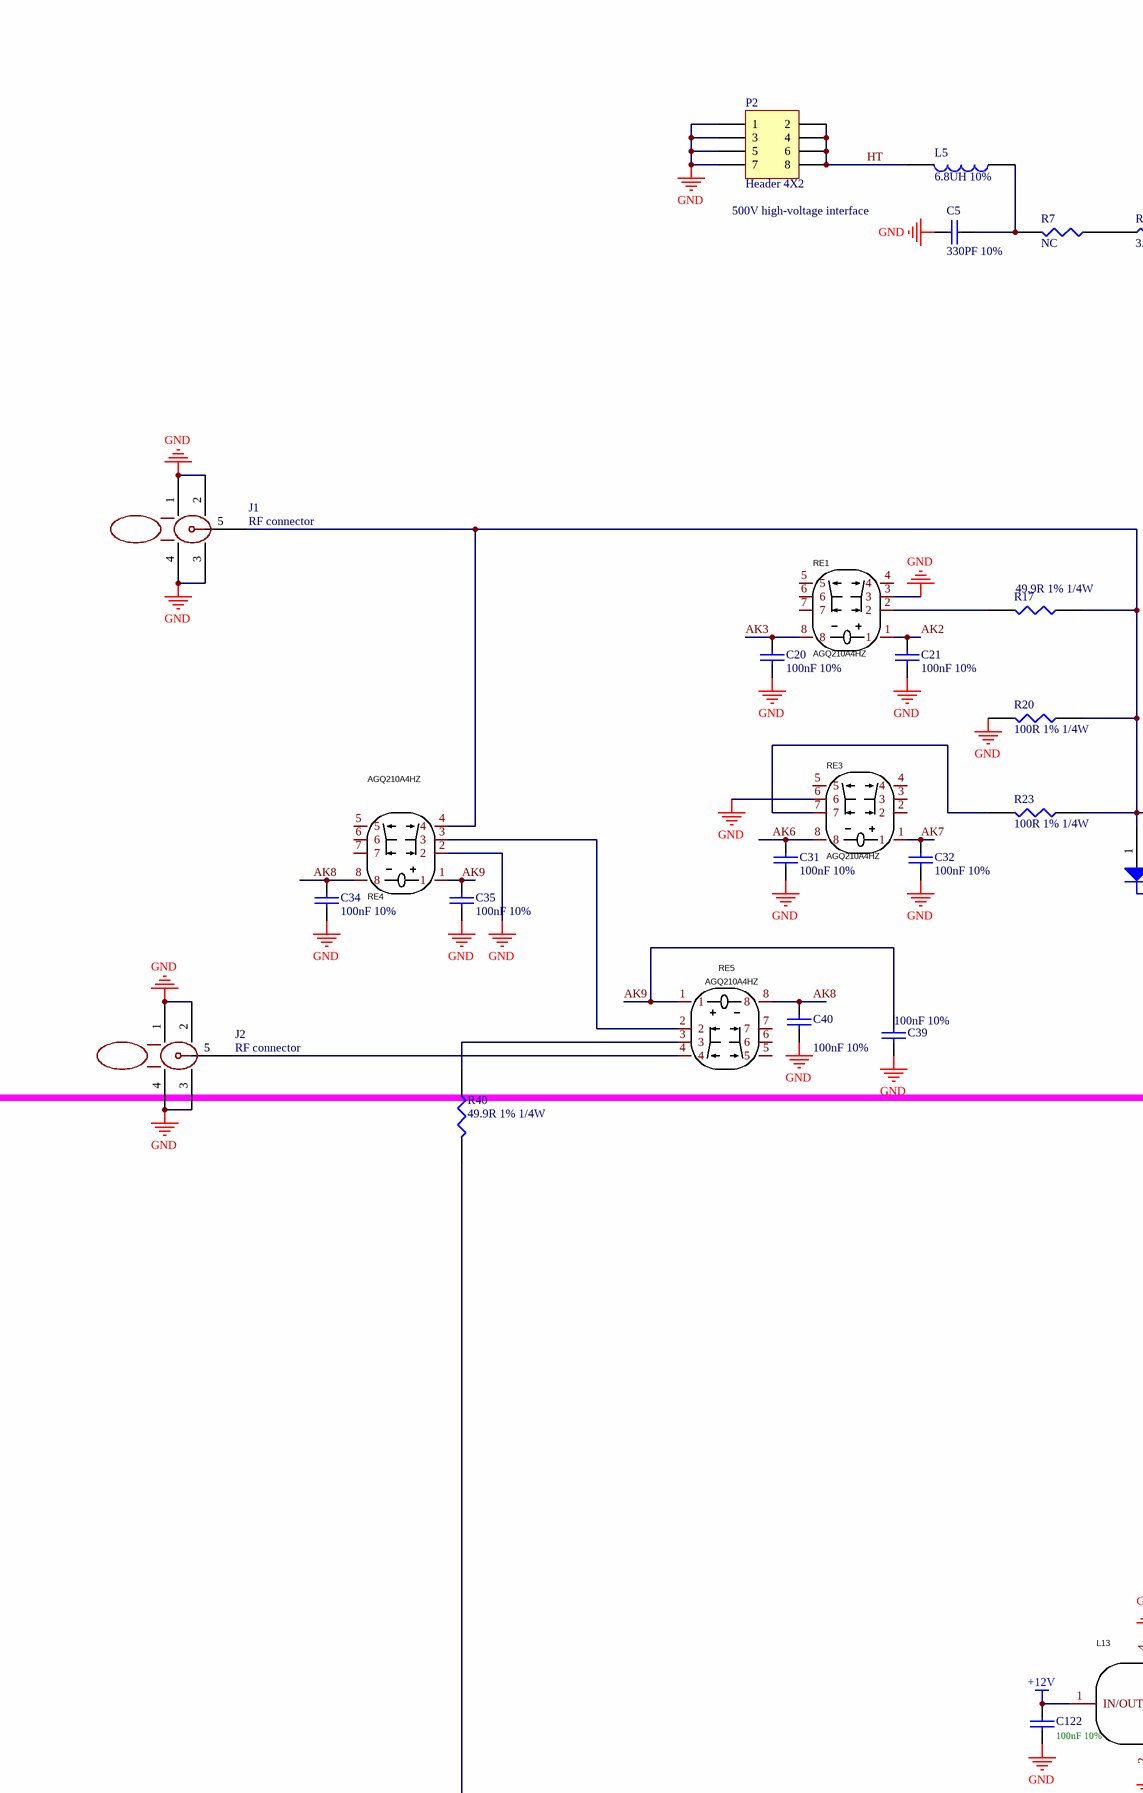
[diagram p0: PCBE109560-12.SchDoc, top left]
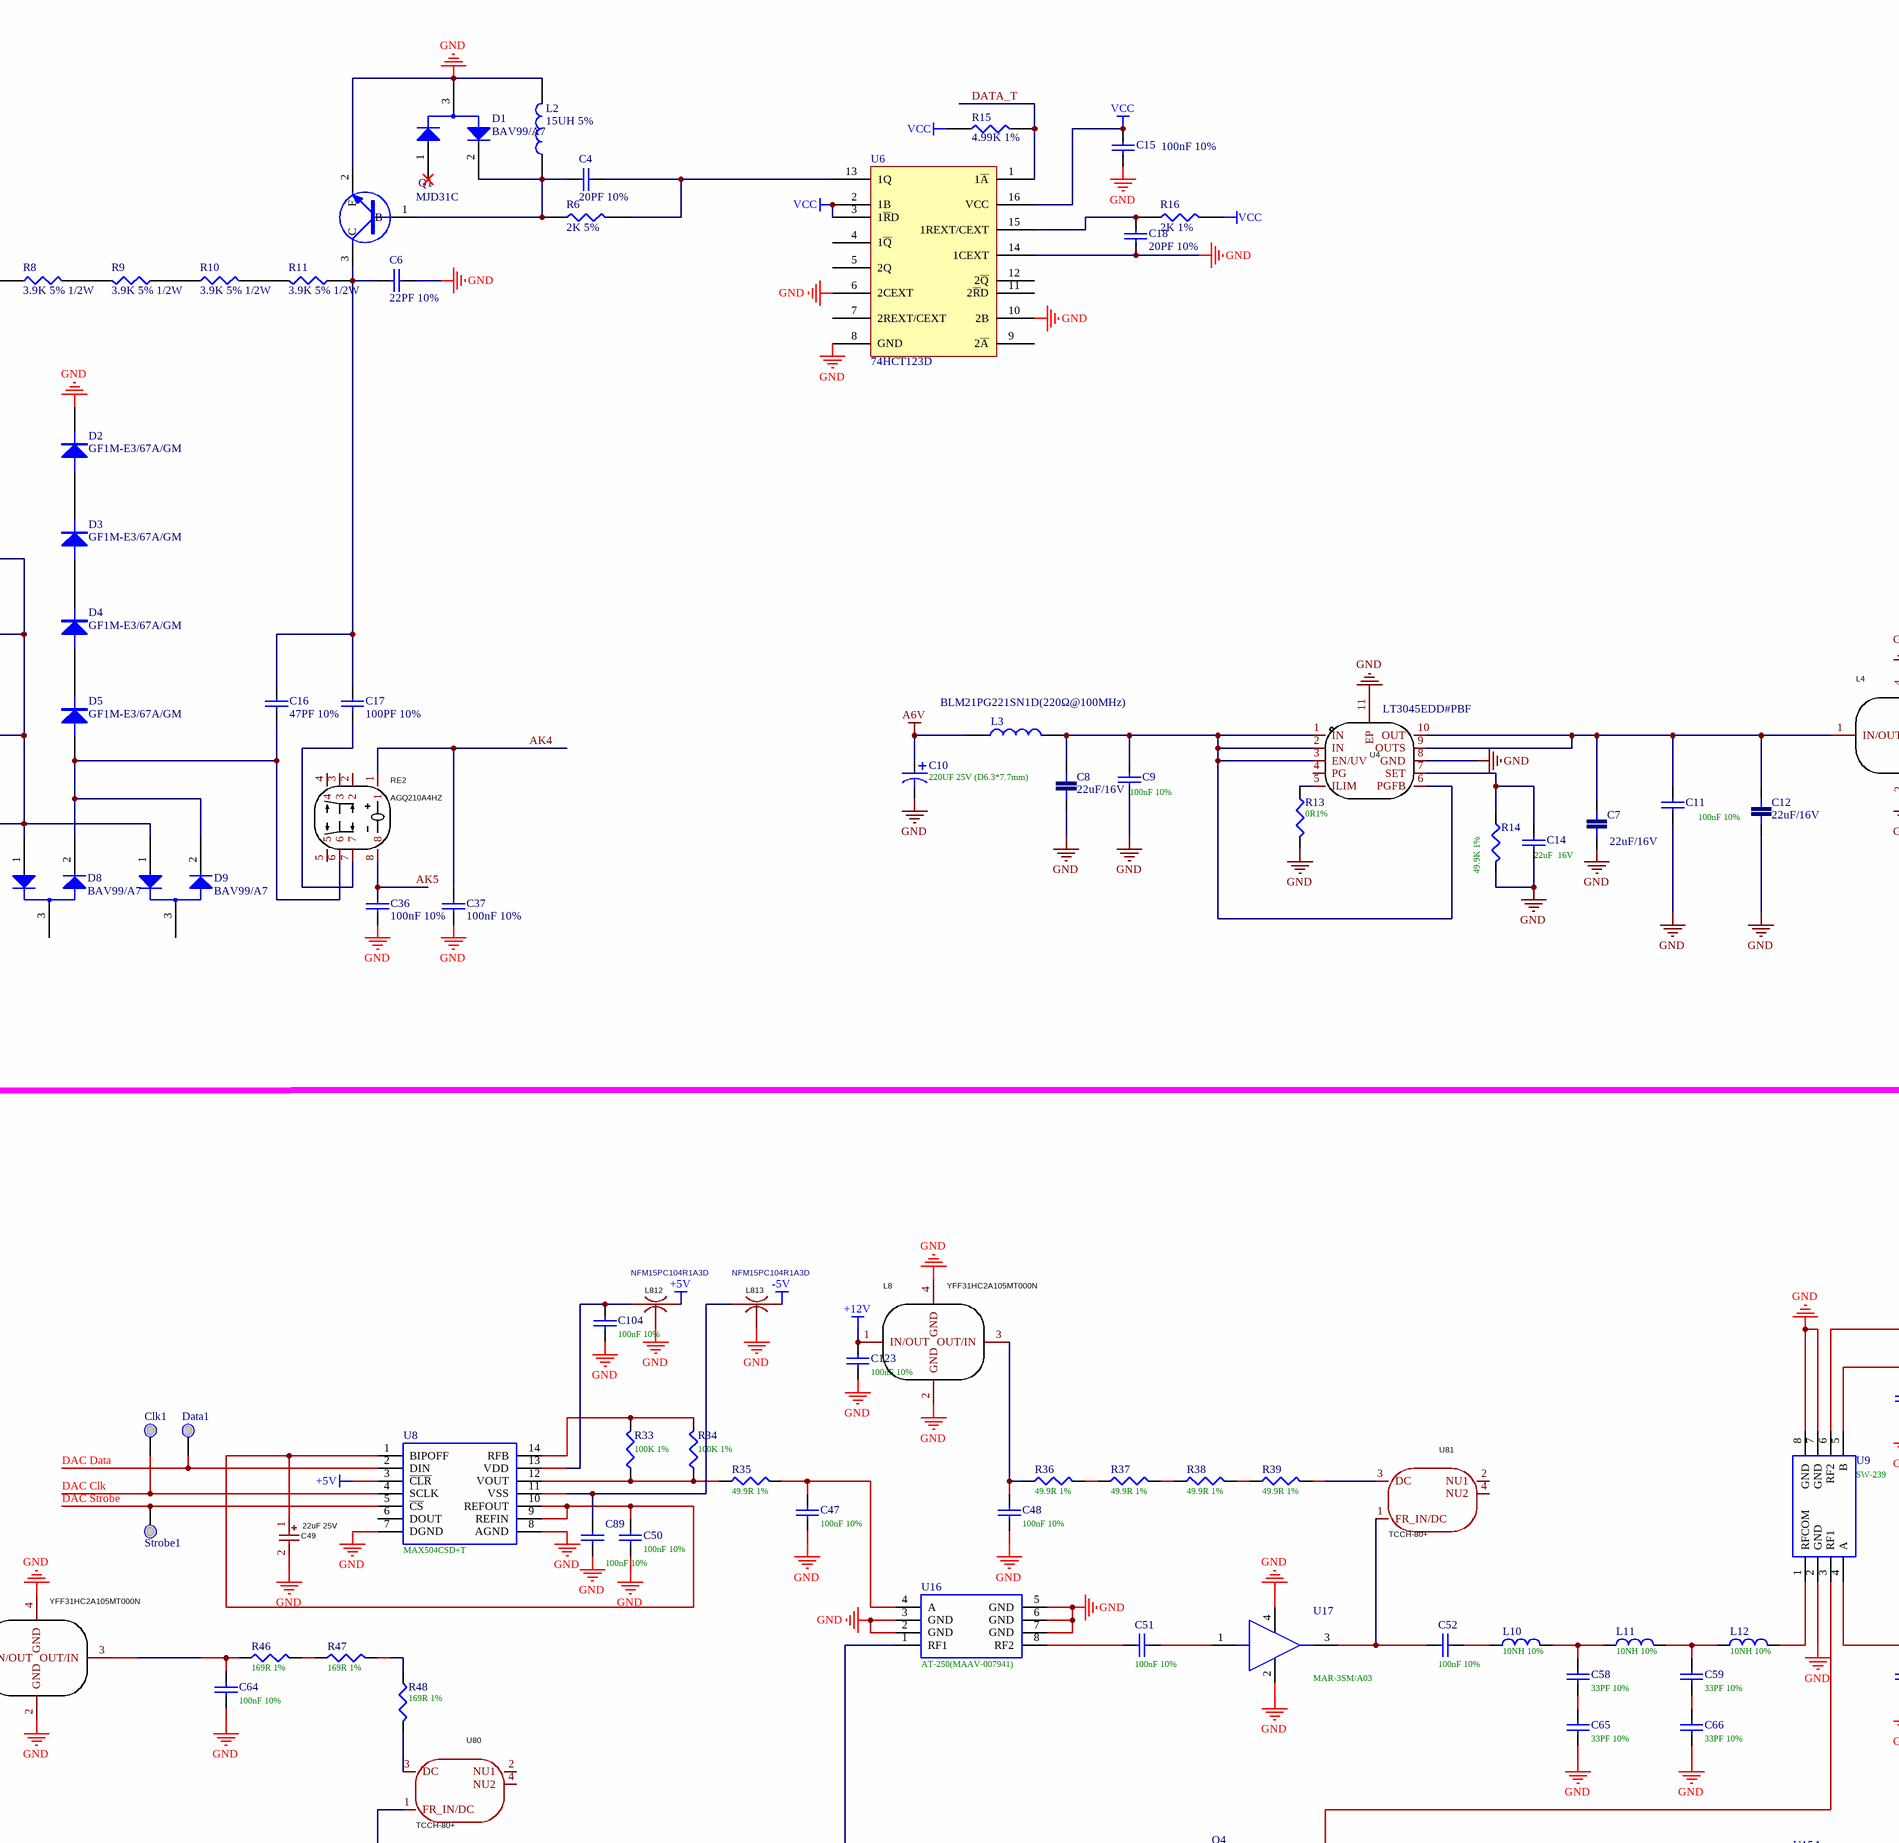
[diagram p1: PCBE109560-12.SchDoc, top middle]
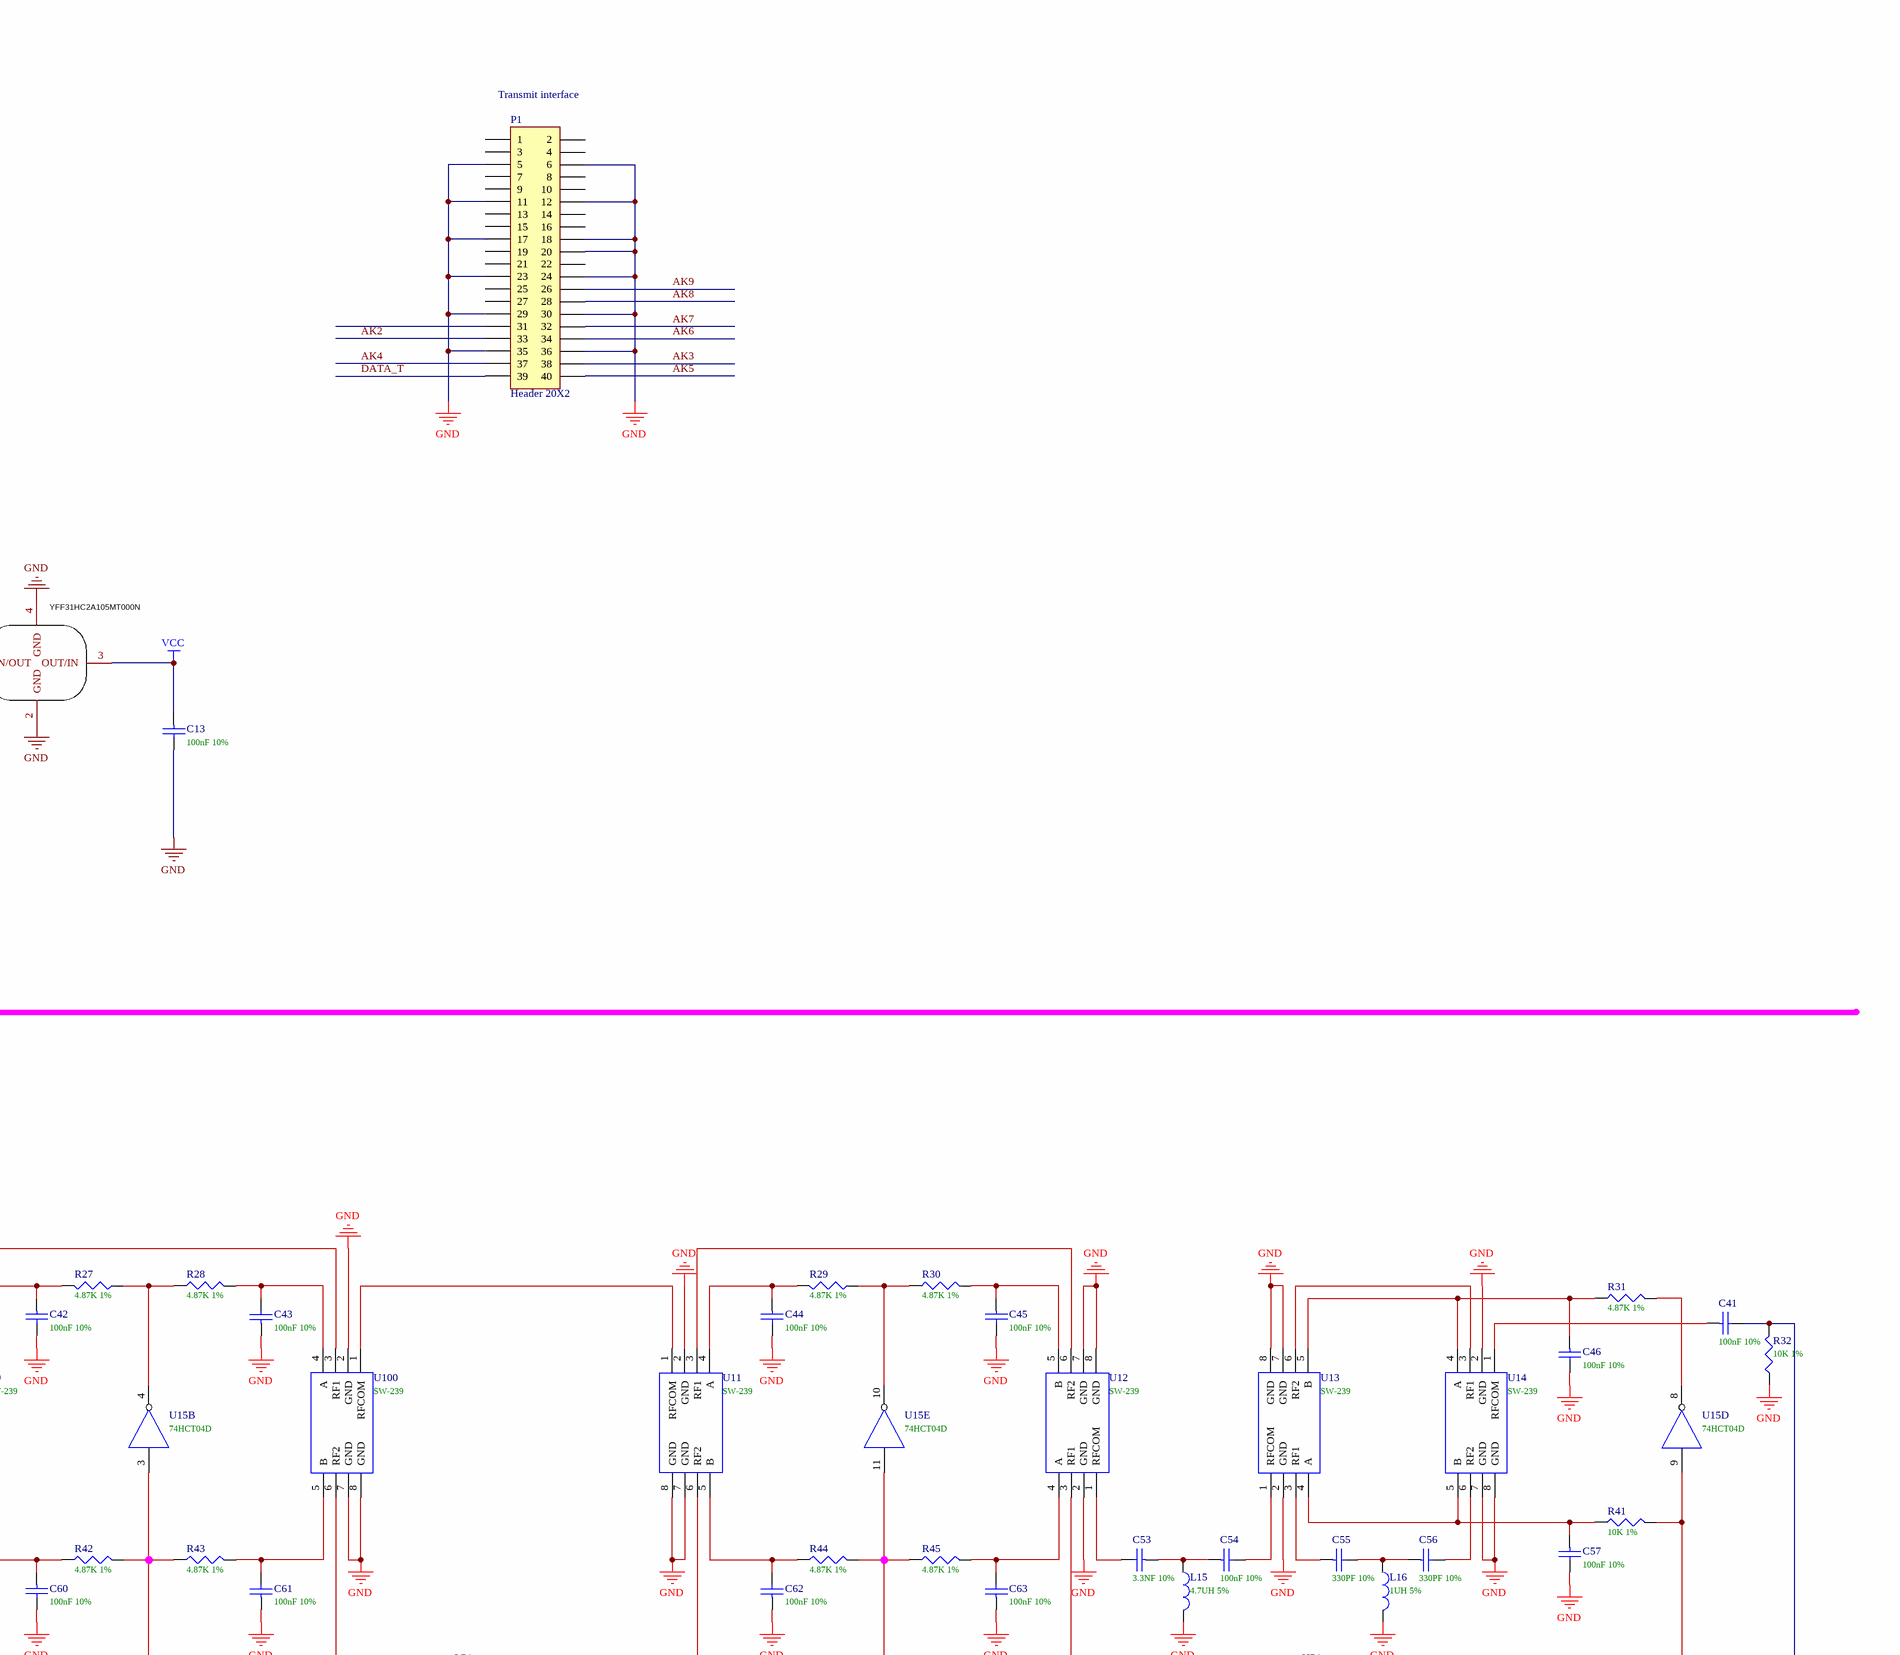
[diagram p2: PCBE109560-12.SchDoc, top right]
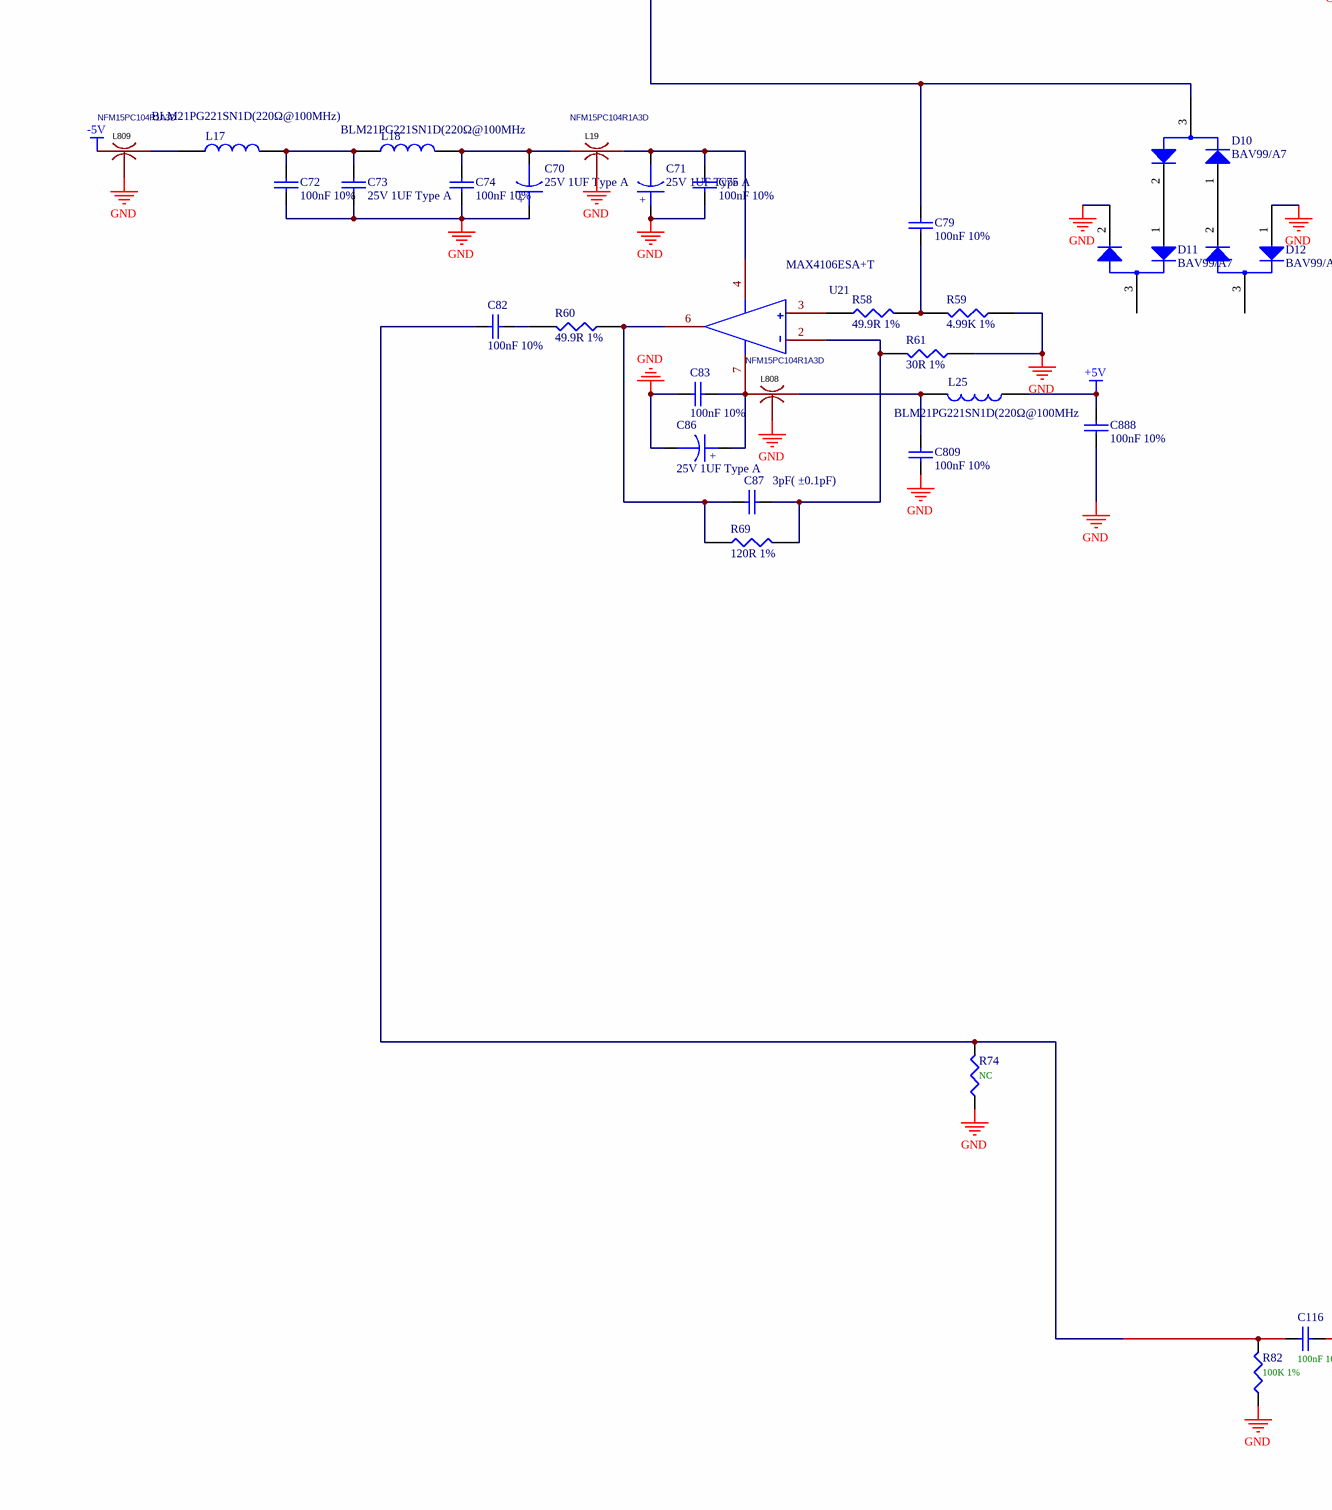
[diagram p3: PCBE109560-12.SchDoc, bottom left]
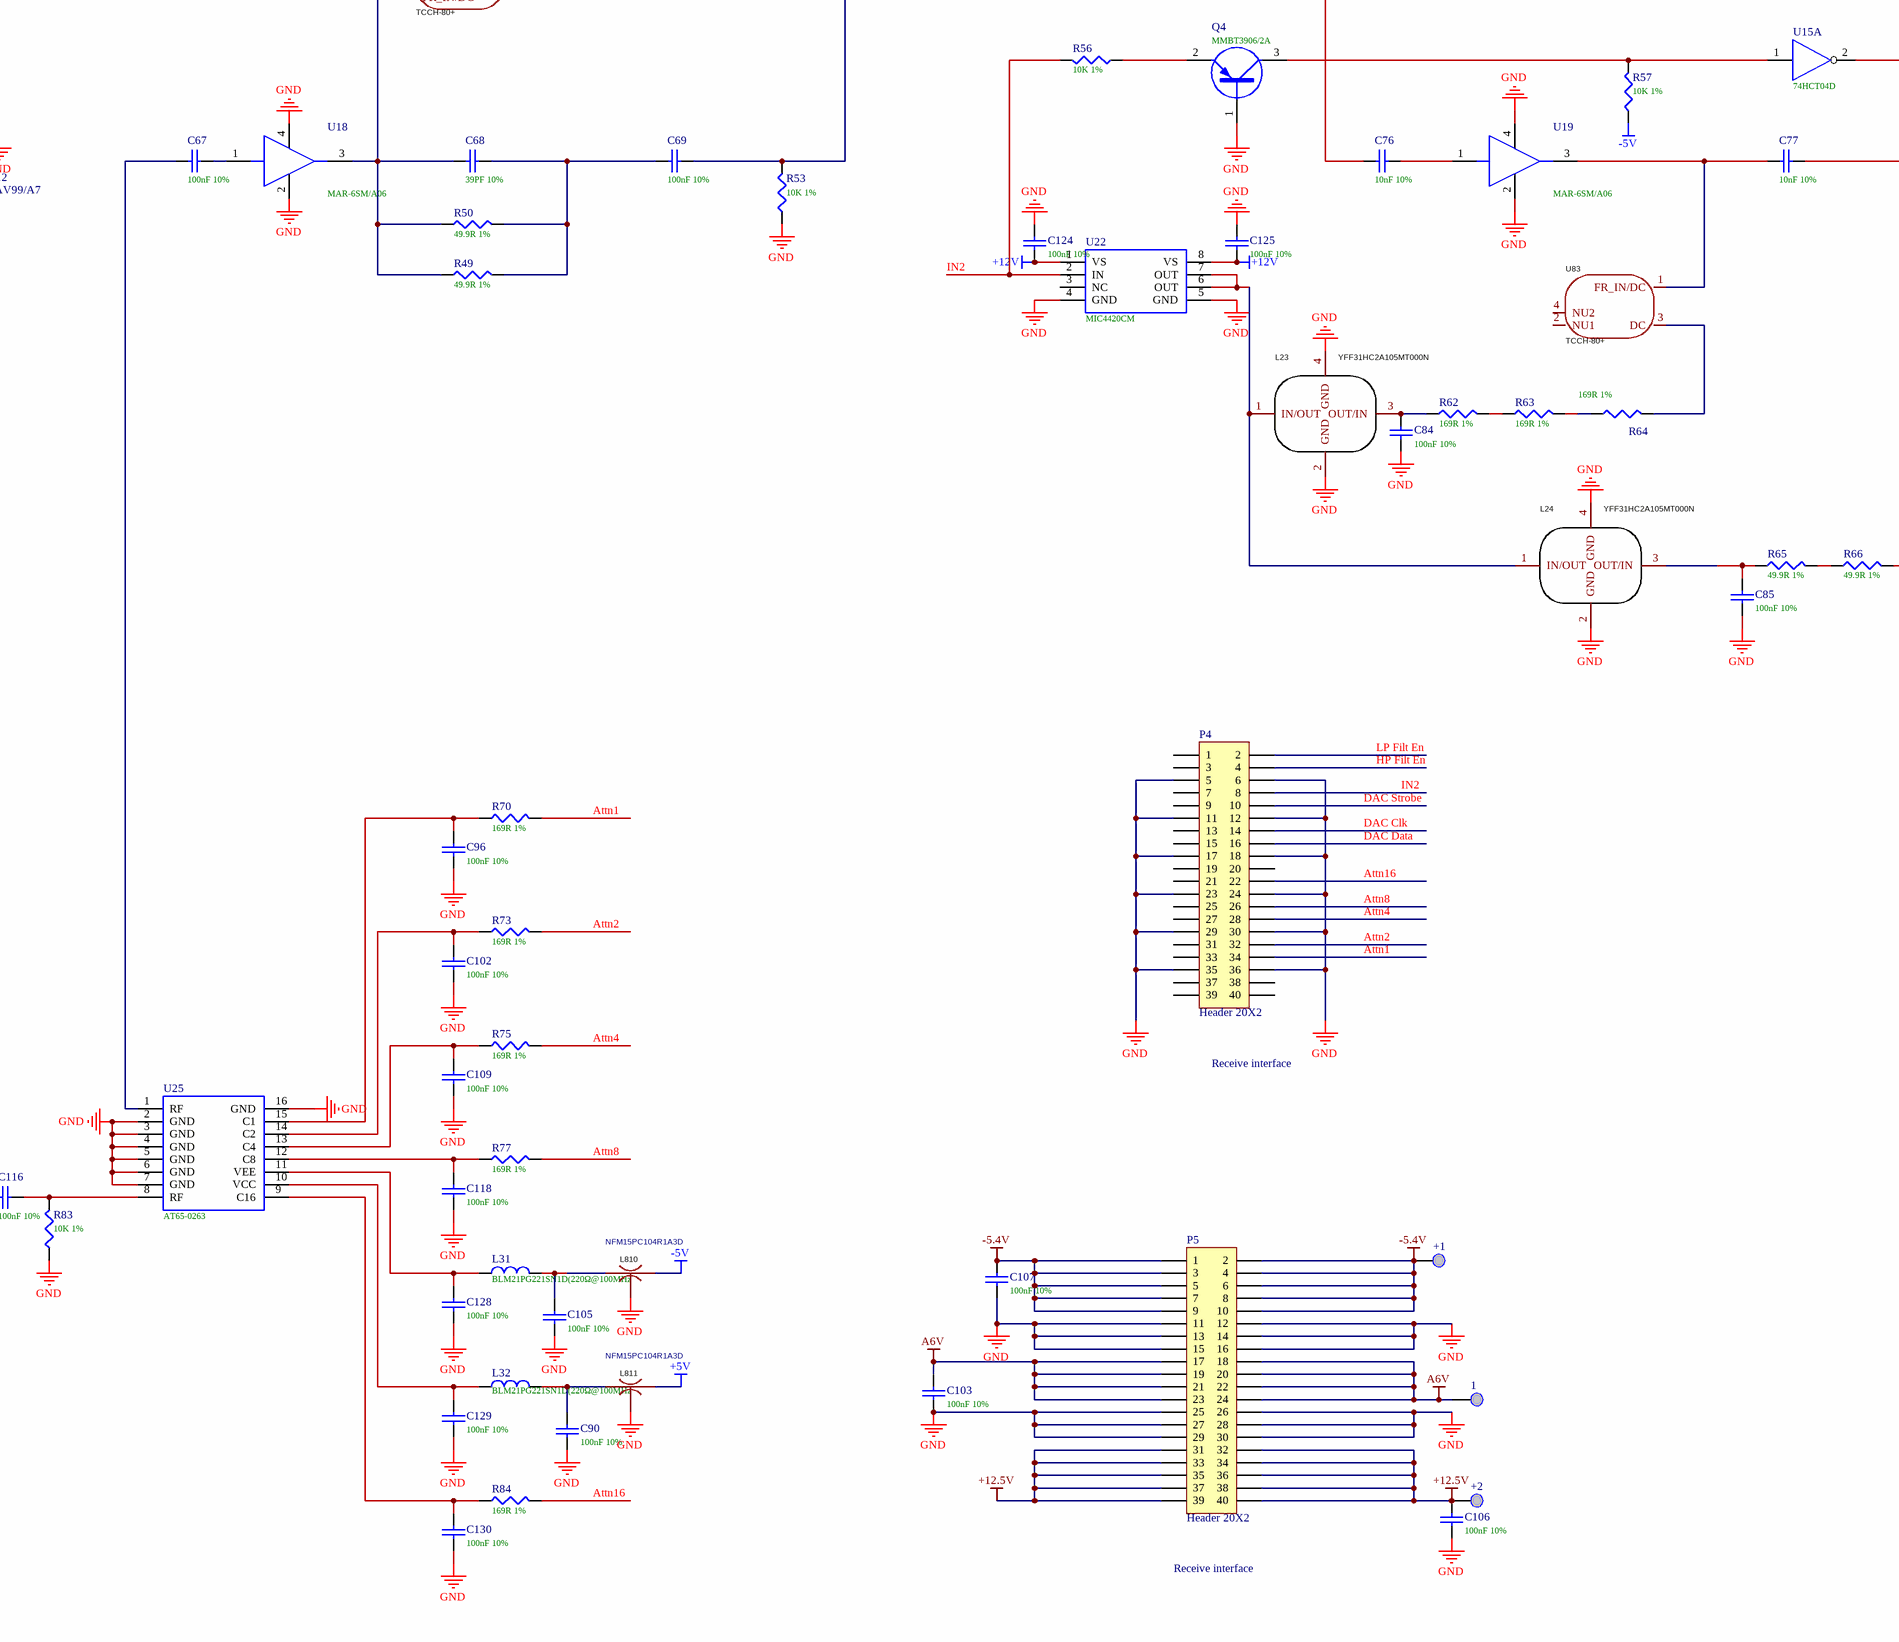
[diagram p4: PCBE109560-12.SchDoc, bottom middle]
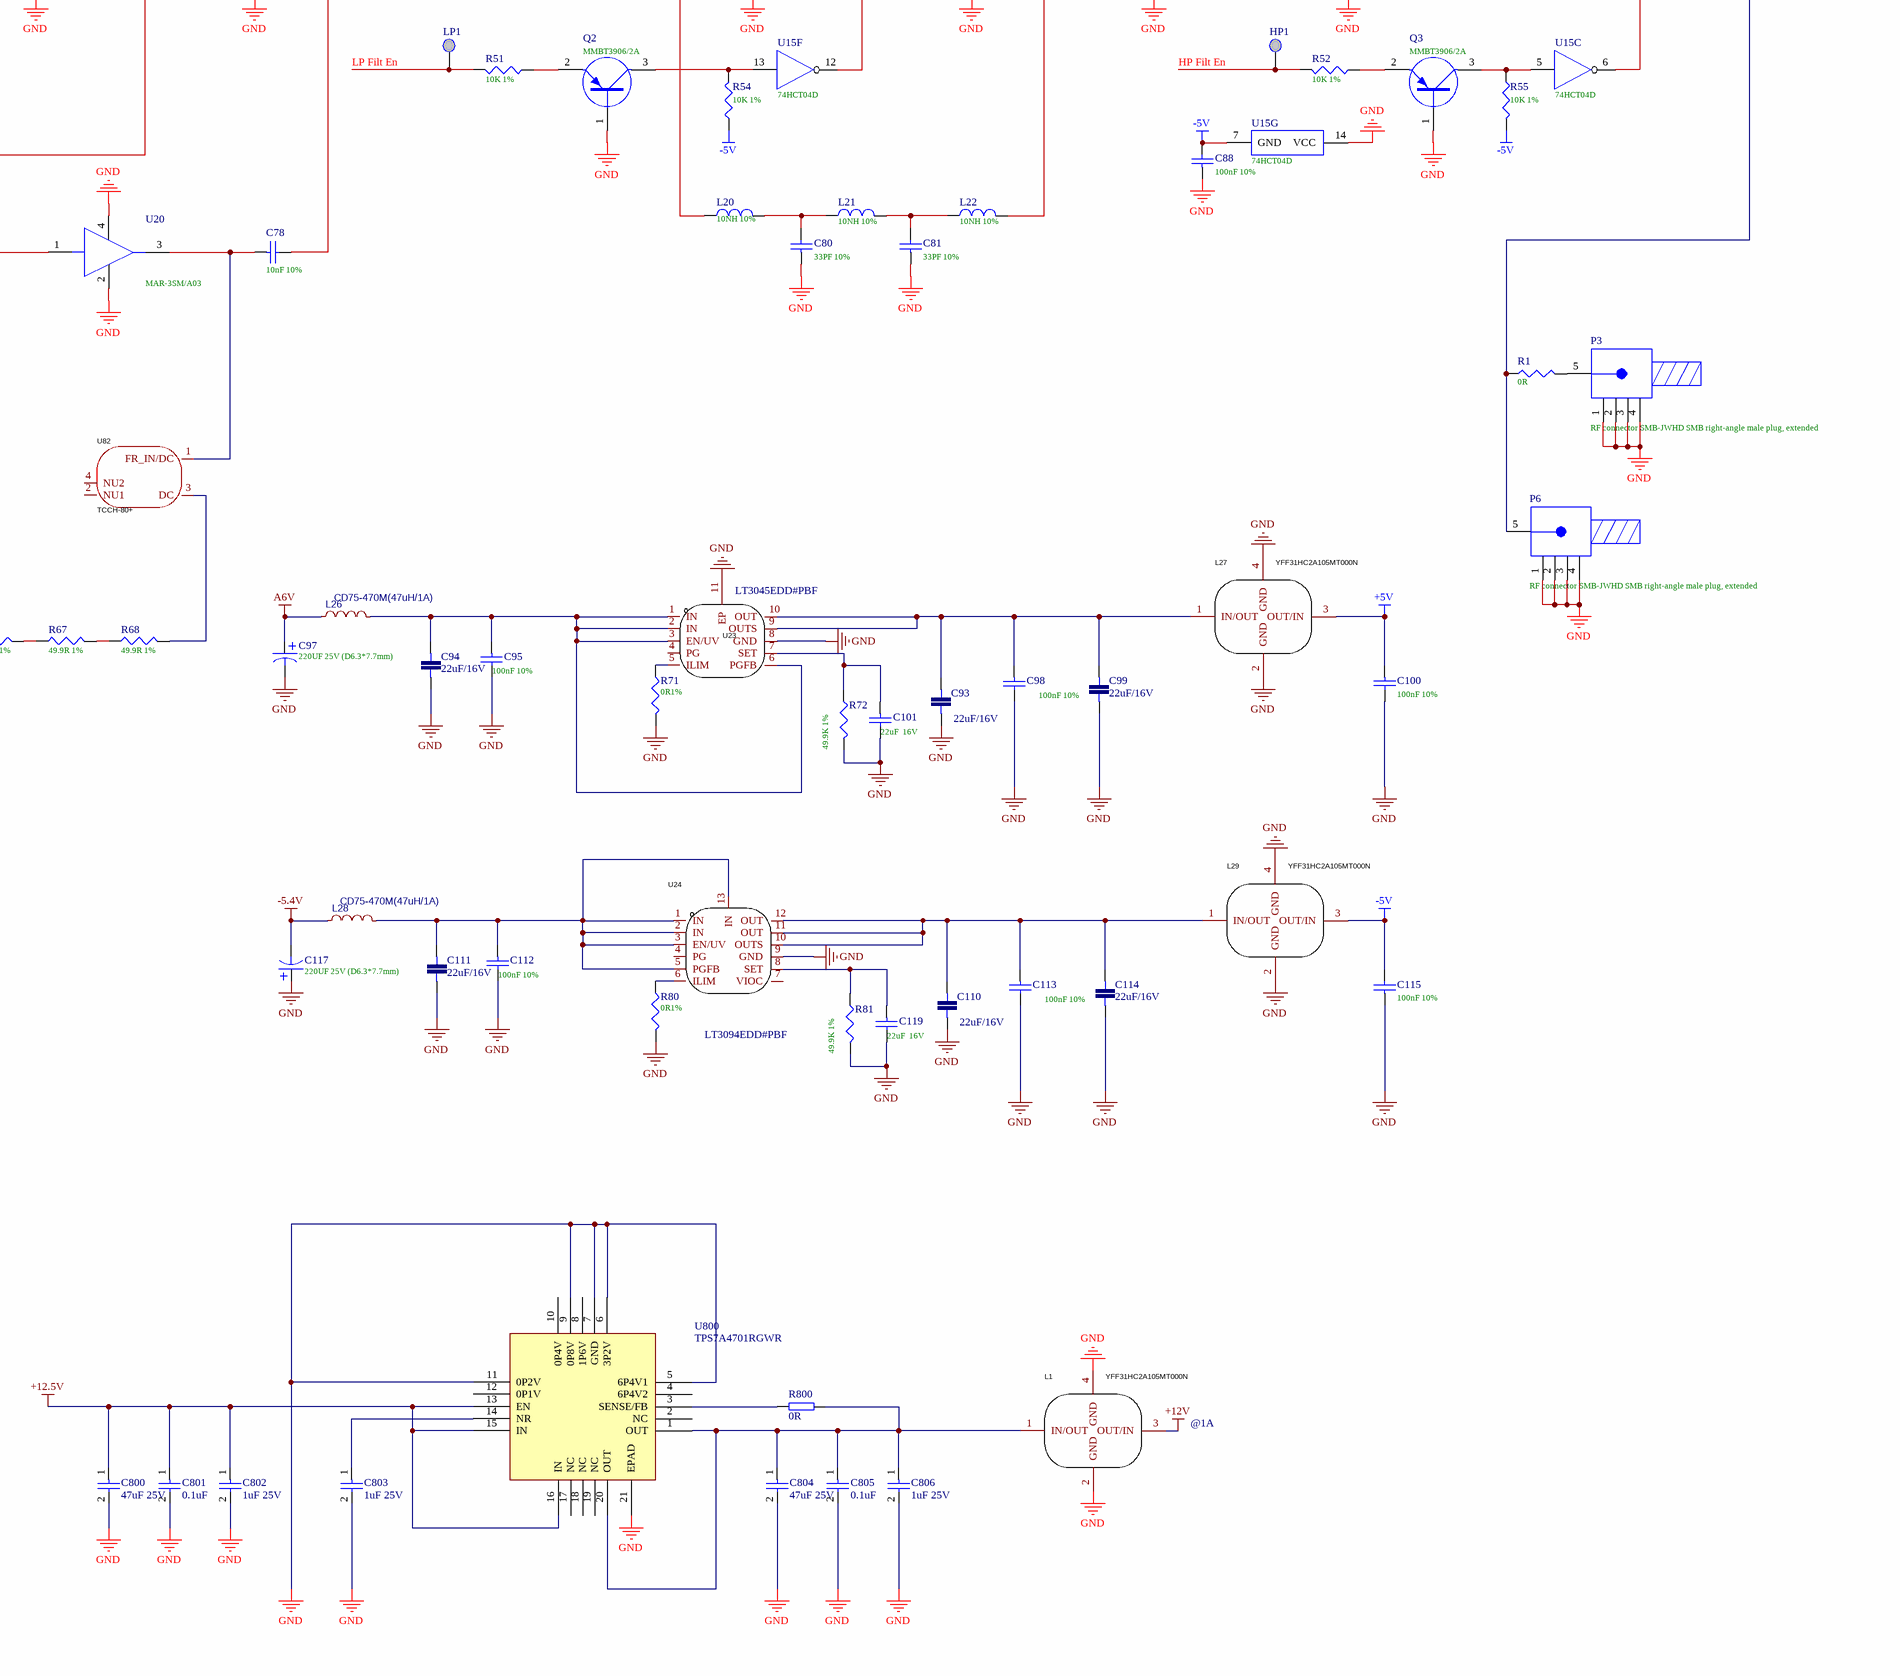
[diagram p5: PCBE109560-12.SchDoc, bottom right]
# Altium project MISC109560-2.PrjPcb (part 1 of 2)
1 sheet, 280 parts. Net scope: global (net labels, ports and power ports of the same name join across sheets).
Board file: MISC109560.PcbDoc